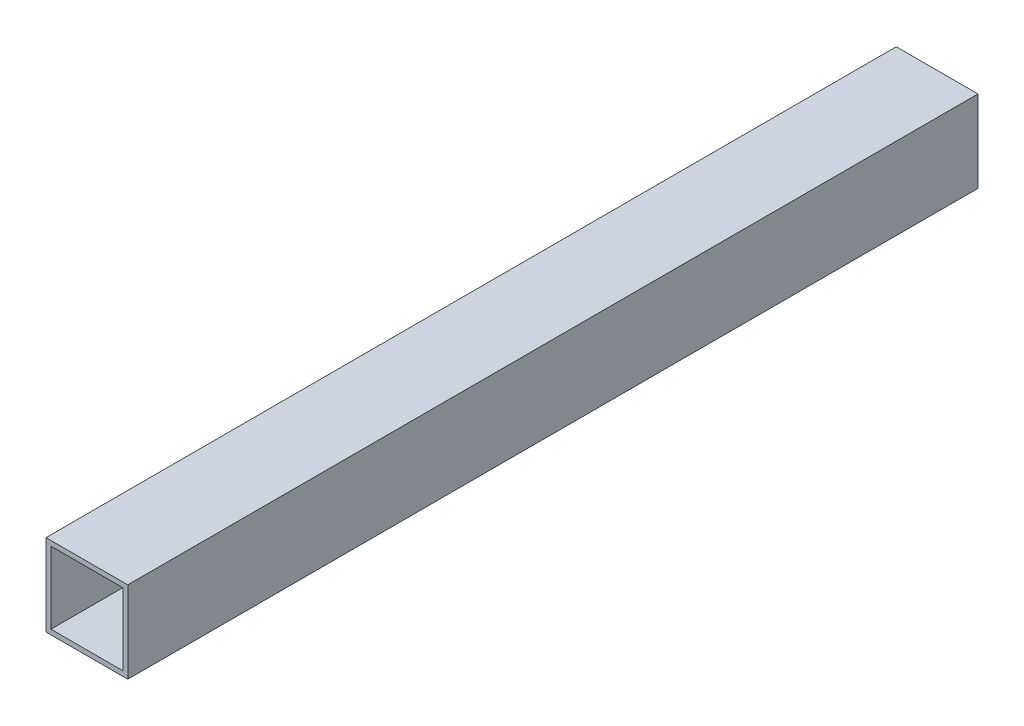
SolidWorks part; units mm, degrees
ref_plane "前视基准面" through (0, 0, 0) normal (0, 0, 1) x (1, 0, 0)
ref_plane "上视基准面" through (0, 0, 0) normal (0, 1, 0) x (1, 0, 0)
ref_plane "右视基准面" through (0, 0, 0) normal (1, 0, 0) x (0, 0, -1)
sketch "草图1" plane through (0, 0, 0) normal (0, 0, 1) x (1, 0, 0)
  line L0 (0, 0) -> (50, 0)
  line L1 (50, 0) -> (50, 50)
  line L2 (50, 50) -> (0, 50)
  line L3 (0, 50) -> (0, 0)
  line L4 (3, 3) -> (47, 3)
  line L5 (47, 3) -> (47, 47)
  line L6 (47, 47) -> (3, 47)
  line L7 (3, 47) -> (3, 3)
  dimension "D1" = 3
extrude "凸台-拉伸1" add sketch "草图1" along normal blind 520
sketch "草图2" plane through (0, 0, 520) normal (0, 0, 1) x (1, 0, 0)
  line L4 (3, 47) -> (47, 47)
  line L5 (47, 47) -> (47, 3)
  line L6 (47, 3) -> (3, 3)
  line L7 (3, 3) -> (3, 47)
  line L8 (0, 50) -> (0, 0)
  line L9 (0, 0) -> (50, 0)
  line L10 (50, 0) -> (50, 50)
  line L11 (50, 50) -> (0, 50)
  line L12 (0, 50) -> (0, 0)
  line L13 (0, 0) -> (50, 0)
  line L14 (50, 0) -> (50, 50)
  line L15 (50, 50) -> (0, 50)
  dimension "D1" = 0
extrude "凸台-拉伸2" add sketch "草图2" along normal blind 70
sketch "草图3" plane through (0, 0, 590) normal (0, 0, 1) x (1, 0, 0)
  line L8 (50, 50) -> (0, 50)
  line L9 (0, 50) -> (0, 0)
  line L10 (0, 0) -> (50, 0)
  line L11 (50, 0) -> (50, 50)
  line L12 (50, 50) -> (0, 50)
  line L13 (0, 50) -> (0, 0)
  line L14 (0, 0) -> (50, 0)
  line L15 (50, 0) -> (50, 50)
  dimension "D1" = 0
extrude "切除-拉伸1" cut sketch "草图3" against normal blind 70
